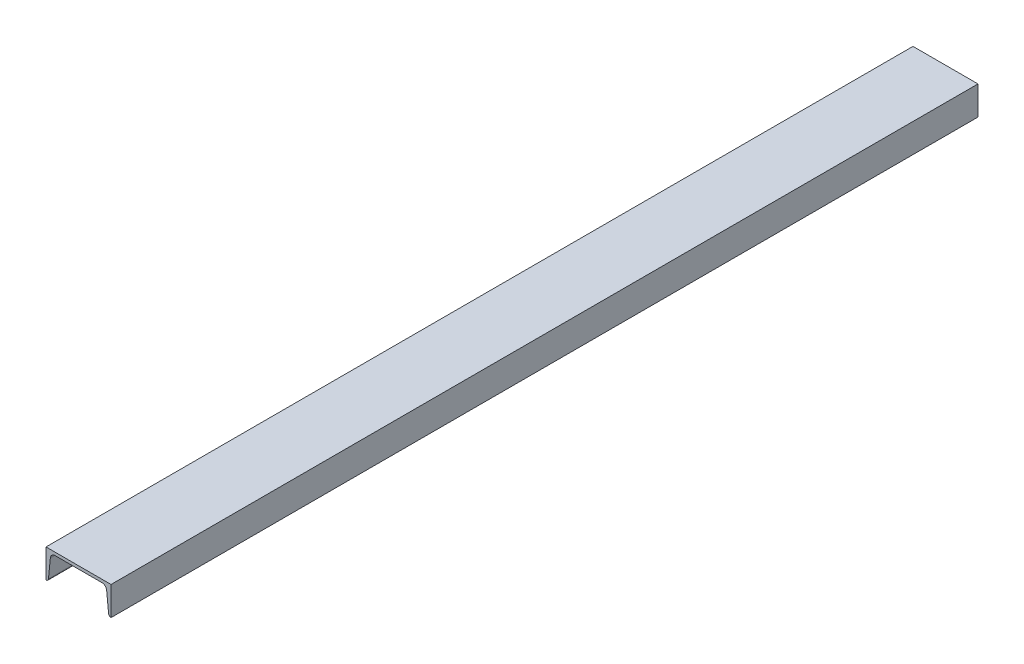
SolidWorks part; units mm, degrees
ref_plane "Front Plane" through (0, 0, 0) normal (0, 0, 1) x (1, 0, 0)
ref_plane "Top Plane" through (0, 0, 0) normal (0, 1, 0) x (1, 0, 0)
ref_plane "Right Plane" through (0, 0, 0) normal (1, 0, 0) x (0, 0, -1)
sketch "Sketch 1" plane through (0, 0, 0) normal (0, 0, 1) x (1, 0, 0)
  line L0 (0, 50.9167) -> (0, -84.5) construction
  line L1 (-68.9722, 0) -> (76.5556, 0) construction
  line L2 (60, 0) -> (-60, 0)
  line L3 (-60, 0) -> (-60, -53)
  line L4 (-55.5223, -48.9477) -> (-51.9884, -13.6046)
  line L5 (-43.033, -5.5) -> (43.033, -5.5)
  line L8 (55.5223, -48.9477) -> (51.9884, -13.6046)
  line L9 (60, 0) -> (60, -53)
  arc A0 (-60, -53) -> (-55.5223, -48.9477) centre (-60, -48.5) ccw
  arc A1 (60, -53) -> (55.5223, -48.9477) centre (60, -48.5) cw
  arc A2 (51.9884, -13.6046) -> (43.033, -5.5) centre (43.033, -14.5) ccw
  arc A3 (-51.9884, -13.6046) -> (-43.033, -5.5) centre (-43.033, -14.5) cw
  point P15 (0, 0)
  point P17 (0, -5.5)
  point P21 (51.178, -5.5)
  point P24 (-51.178, -5.5)
  dimension "D3" = 4.5
  dimension "D5" = 9
  dimension "D1" = 120
  dimension "D2" = 5.5
  dimension "D4" = 53
  dimension "D6" = 5.71
extrude "Boss-Extrude 1" add sketch "Sketch 1" along normal mid plane 1600
